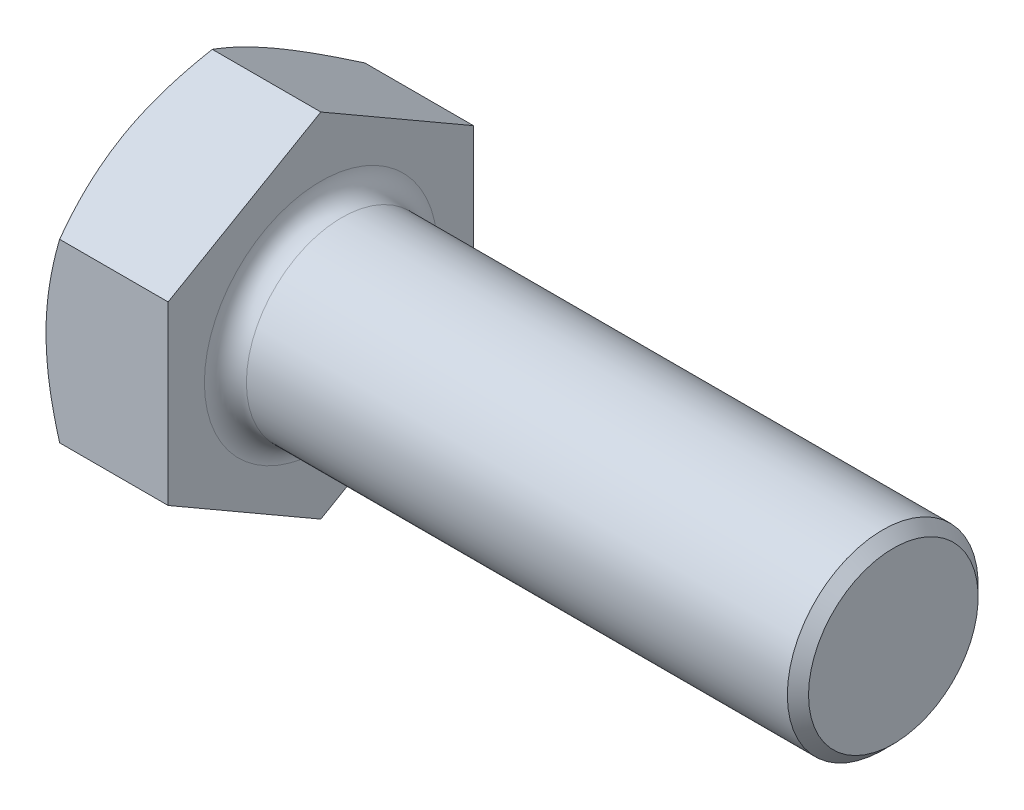
SolidWorks part; units mm, degrees
material "Q235"
ref_plane "Front Plane" through (0, 0, 0) normal (0, 0, 1) x (1, 0, 0)
ref_plane "Top Plane" through (0, 0, 0) normal (0, 1, 0) x (1, 0, 0)
ref_plane "Right Plane" through (0, 0, 0) normal (1, 0, 0) x (0, 0, -1)
sketch "Sketch 1" plane through (0, 0, 0) normal (0, 0, 1) x (1, 0, 0)
  line L0 (0, 0) -> (36.4, 0) construction
  line L1 (0, 0) -> (0, 8.795)
  line L2 (0, 8.795) -> (6.4, 8.795)
  line L3 (6.4, 8.795) -> (6.4, 0)
  line L4 (6.4, 5) -> (36.4, 5)
  line L5 (36.4, 5) -> (36.4, 0)
  line L6 (0, 8) -> (0.459, 8.795)
  line L7 (33.4, 5) -> (33.4, 0)
  line L8 (10.9, 5) -> (10.9, 0)
  line L9 (6.4, 4.5129) -> (36.4, 4.5129)
  line L10 (36.4, 4.1881) -> (6.4, 4.1881)
  line L11 (5.8, 7.735) -> (6.4, 7.135)
  line L12 (5.8, 8.795) -> (5.8, 0)
  line L13 (6.3, 7.235) -> (6.3, 0) construction
  arc A0 (6.4, 6.1) -> (7.5, 5) centre (7.5, 6.1) ccw
  point P12 (34.9, 0)
  point P13 (2.23, 8.795)
  point P14 (6.4, 6.1)
  point P24 (6.4, 7.235)
  dimension "D1" = 0.1
  dimension "r" = 1.1
  dimension "k" = 6.4
  dimension "D2" = 45
  dimension "β" = 30
  dimension "e" = 17.59
  dimension "s" = 16
  dimension "d" = 10
  dimension "l" = 30
  dimension "D52" = 3
  dimension "P" = 1.5
  dimension "kw" = 4.17
  dimension "da" = 12.2
  dimension "a" = 4.5
  dimension "ds" = 9.0258
  dimension "D61" = 8.3763
  dimension "dw" = 14.47
  dimension "c" = 0.6
sketch "Sketch2" plane through (0, 0, 0) normal (1, 0, 0) x (0, 0, -1)
  line L1 (0, 9.2376) -> (-8, 4.6188)
  line L2 (-8, 4.6188) -> (-8, -4.6188)
  line L3 (-8, -4.6188) -> (0, -9.2376)
  line L4 (0, -9.2376) -> (8, -4.6188)
  line L5 (8, -4.6188) -> (8, 4.6188)
  line L6 (8, 4.6188) -> (0, 9.2376)
  circle A0 centre (0, 0) radius 8 construction
sketch "Sketch3" plane through (0, 0, 0) normal (1, 0, 0) x (0, 0, -1)
  line L0 (8, 4.6188) -> (0, 9.2376) construction
  line L1 (0, 9.2376) -> (-8, 4.6188) construction
  line L2 (-8, 4.6188) -> (-8, -4.6188) construction
  line L3 (8, -4.6188) -> (8, 4.6188) construction
  line L4 (0, -9.2376) -> (8, -4.6188) construction
  line L5 (-8, -4.6188) -> (0, -9.2376) construction
  line L6 (8, 4.6188) -> (0, 9.2376)
  line L7 (0, 9.2376) -> (-8, 4.6188)
  line L8 (-8, 4.6188) -> (-8, -4.6188)
  line L9 (8, -4.6188) -> (8, 4.6188)
  line L10 (0, -9.2376) -> (8, -4.6188)
  line L11 (-8, -4.6188) -> (0, -9.2376)
extrude "Boss-Extrude1" add sketch "Sketch3" along normal up to vertex (6.4 mm away) up to point (6.4, 8.795, 0)
sketch "Sketch4" plane through (0, 0, 0) normal (-1, 0, 0) x (0, 0, 1)
  circle A0 centre (0, 0) radius 8 construction
  circle A1 centre (0, 0) radius 8
  circle A2 centre (0, 0) radius 17.59
  dimension "D1" = 35.18
extrude "Cut-Extrude1" cut sketch "Sketch4" against normal blind 0.8 draft 60
sketch "Sketch5" plane through (0, 0, 0) normal (0, 0, 1) x (1, 0, 0)
  line L0 (6.4, 5) -> (36.4, 5) construction
  line L1 (36.4, 5) -> (36.4, 0) construction
  line L2 (0, 0) -> (36.4, 0) construction
  line L3 (7.5, 5) -> (36.4, 5)
  line L4 (36.4, 5) -> (36.4, 0)
  line L5 (6.4, 0) -> (36.4, 0)
  line L6 (6.4, 6.1) -> (6.4, 0)
  arc A0 (6.4, 6.1) -> (7.5, 5) centre (7.5, 6.1) ccw construction
  arc A1 (6.4, 6.1) -> (7.5, 5) centre (7.5, 6.1) ccw
revolve "Revolve1" add sketch "Sketch5" angle 360 about L5
cosmetic thread "Cosmetic Thread2" parameters "D1"=35.5, "D2"=8.3763
chamfer "Chamfer2" distance 0.5556 angle 45 1 edges at (36.4, 0, 5)
sketch "Sketch7" plane through (0, 0, 0) normal (0, 0, 1) x (1, 0, 0)
  line L0 (6.4, 7.135) -> (5.8, 7.735)
  line L1 (5.8, 7.735) -> (5.8, 17.59)
  line L2 (5.8, 17.59) -> (6.4, 17.59)
  line L3 (6.4, 17.59) -> (6.4, 7.135)
  line L4 (0, 0) -> (36.4, 0) construction
  line L5 (0, 0) -> (36.4, 0) construction
  dimension "D1" = 35.18
revolve "Cut-Revolve1" [suppressed] cut sketch "Sketch7" angle 360 mid plane about L5
sketch "Sketch6" [suppressed] plane through (0, 0, 0) normal (0, 0, 1) x (1, 0, 0)
  line L0 (5.9, 0) -> (5.9, 2.5) construction
  line L1 (5.9, 2.5) -> (13.5, 2.5)
  line L2 (13.5, 2.5) -> (13.5, 0)
  line L3 (5.9, 2.5) -> (4.069, 2.245)
  line L5 (3.5, 2.2402) -> (13.5, 2.2402) construction
  line L6 (3.5, 4.315) -> (3.5, 0) construction
  line L7 (3.5, 2.7402) -> (3.5, 0)
  line L8 (3.5, 0) -> (13.5, 0)
  arc A0 (4.069, 2.245) -> (3.5, 2.7402) centre (4, 2.7402) cw
  arc A1 (3.5, 3) -> (4, 2.5) centre (4, 3) ccw construction
revolve "Revolve2" add sketch "Sketch6" angle 360 about L8
cosmetic thread "Cosmetic Thread1" [suppressed] parameters "D1"=25.5, "D2"=8.3763
chamfer "Chamfer1" [suppressed] distance 0.5556 angle 45
sketch "Sketch8" plane through (0, 0, 0) normal (0, 0, 1) x (1, 0, 0)
  line L0 (6.4, 7.135) -> (5.8, 7.735)
  line L1 (5.8, 7.735) -> (5.8, 17.59)
  line L2 (5.8, 17.59) -> (6.4, 17.59)
  line L3 (6.4, 17.59) -> (6.4, 7.135)
  line L4 (0, 0) -> (36.4, 0) construction
  line L5 (0, 0) -> (36.4, 0) construction
  dimension "D1" = 35.18
revolve "Cut-Revolve2" [suppressed] cut sketch "Sketch8" angle 360 mid plane about L5
